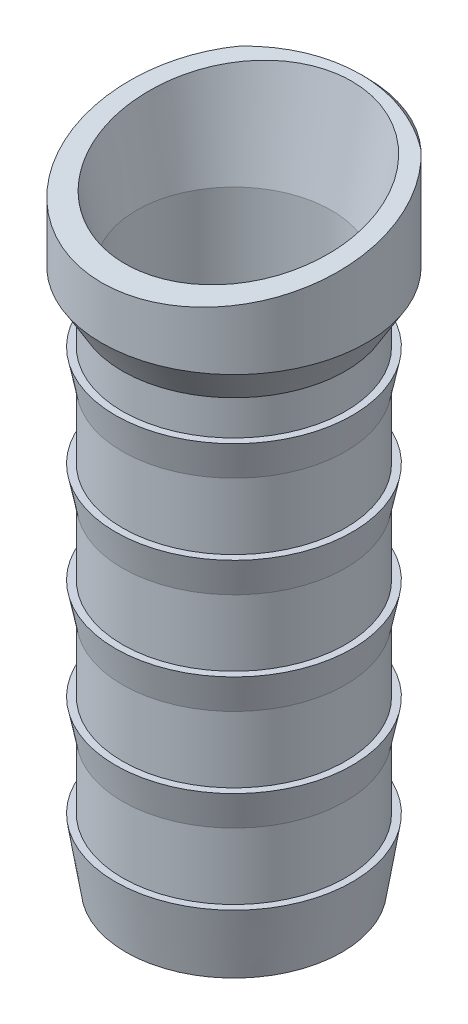
from build123d import *

# Parameters (mm, degrees)
SKETCH_2_R          = 28
CUT_EXTRUDE_1_DEPTH = 185
SKETCH_4_R          = 34
SKETCH_3_R          = 28
CUT_EXTRUDE_2_DEPTH = 50


with BuildPart() as part:
    # 草图1 → 旋转1 (revolve)
    with BuildSketch(Plane.XY, mode=Mode.PRIVATE) as revolve_1_sk:
        Polygon((0, 92.5), (0, -92.5), (31, -92.5), (34, -73.5), (32, -73.5), (32, -54.5), (34, -44.5), (32, -44.5), (32, -25.5), (34, -15.5), (32, -15.5), (32, 3.5), (34, 13.5), (32, 13.5), (32, 32.5), (34, 42.5), (32, 42.5), (32, 52.5), (38, 62.5), (38, 90.5), (36, 92.5), align=None)
    revolve(revolve_1_sk.sketch.rotate(Axis((0, 92.5, 0), (0, -1, 0)), 90), axis=Axis((0, 92.5, 0), (0, -1, 0)))

    # 草图2 → 切除-拉伸1 (cut)
    with BuildSketch(Plane(origin=(0, 92.5, 0), x_dir=(1, 0, 0), z_dir=(0, 1, 0))):
        with Locations(Location((0, 0, 0), (0, 0, 270))):
            Circle(SKETCH_2_R)
    extrude(amount=-CUT_EXTRUDE_1_DEPTH, mode=Mode.SUBTRACT)

    # 草图4 → 切除-放样1 section 0
    with BuildSketch(Plane(origin=(0, 92.5, 0), x_dir=(1, 0, 0), z_dir=(0, 1, 0))):
        Circle(SKETCH_4_R)
    # 草图3 → 切除-放样1 section 1
    with BuildSketch(Plane(origin=(0, 62.5, 0), x_dir=(-1, 0, 0), z_dir=(0, 1, 0))):
        Circle(SKETCH_3_R)
    loft(mode=Mode.SUBTRACT)

    # 草图5 → 切除-拉伸2 (cut, symmetric)
    with BuildSketch(Plane(origin=(0, 0, 0), x_dir=(0, 0, -1), z_dir=(1, 0, 0))):
        Polygon((-38, 77.5), (38, 92.5), (-38, 92.5), align=None)
    extrude(amount=CUT_EXTRUDE_2_DEPTH, both=True, mode=Mode.SUBTRACT)


solid = part.part
